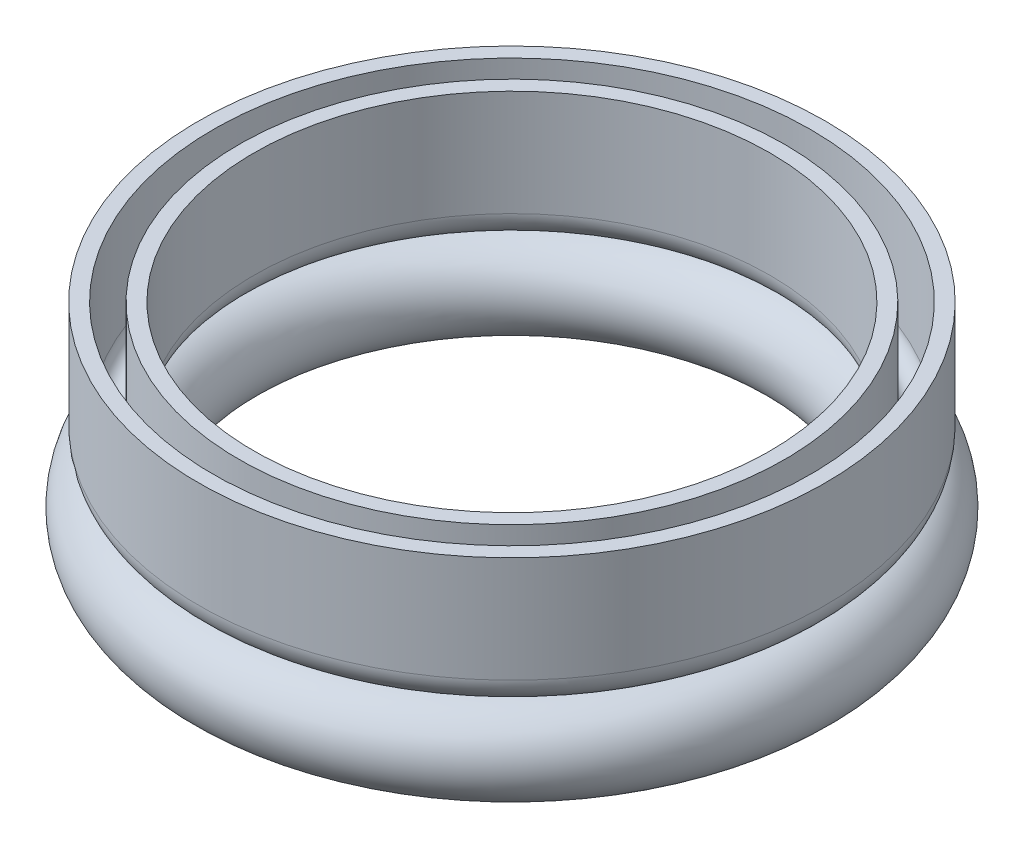
from build123d import *

# Parameters (mm, degrees)
SKETCH3_R   = 4.75
SKETCH3_R_2 = 3.45


with BuildPart() as part:
    # Sweep1: sweep along a path in Sketch 2_2
    with BuildLine(Plane(origin=(0, 0, 0), x_dir=(1, 0, 0), z_dir=(0, 1, 0))) as sweep1_path:
        CenterArc((31, 0), 31, 0, 360)
    # Sketch1 → Sweep1 (sweep)
    with BuildSketch(Plane.XY):
        with BuildLine():
            Line((-3, 19.25), (-3, 7.75))
            ThreePointArc((-3, 7.75), (0, 4.75), (3, 7.75))
            Line((3, 7.75), (3, 19.25))
            Line((3, 19.25), (1.4, 19.25))
            Line((1.4, 19.25), (1.4, 7.75))
            ThreePointArc((1.4, 7.75), (0, 6.35), (-1.4, 7.75))
            Line((-1.4, 7.75), (-1.4, 19.25))
            Line((-1.4, 19.25), (-3, 19.25))
        make_face()
    sweep(path=sweep1_path.line)


with BuildPart() as body_2:
    # Sweep2: sweep along a path in Sketch 2_2 2
    with BuildLine(Plane(origin=(0, 0, 0), x_dir=(1, 0, 0), z_dir=(0, 1, 0))) as sweep2_path:
        CenterArc((31, 0), 31, 0, 360)
    # Sketch3 → Sweep2 (sweep)
    with BuildSketch(Plane.XY):
        Circle(SKETCH3_R)
        Circle(SKETCH3_R_2, mode=Mode.SUBTRACT)
    sweep(path=sweep2_path.line)


solid = Compound([part.part, body_2.part])
